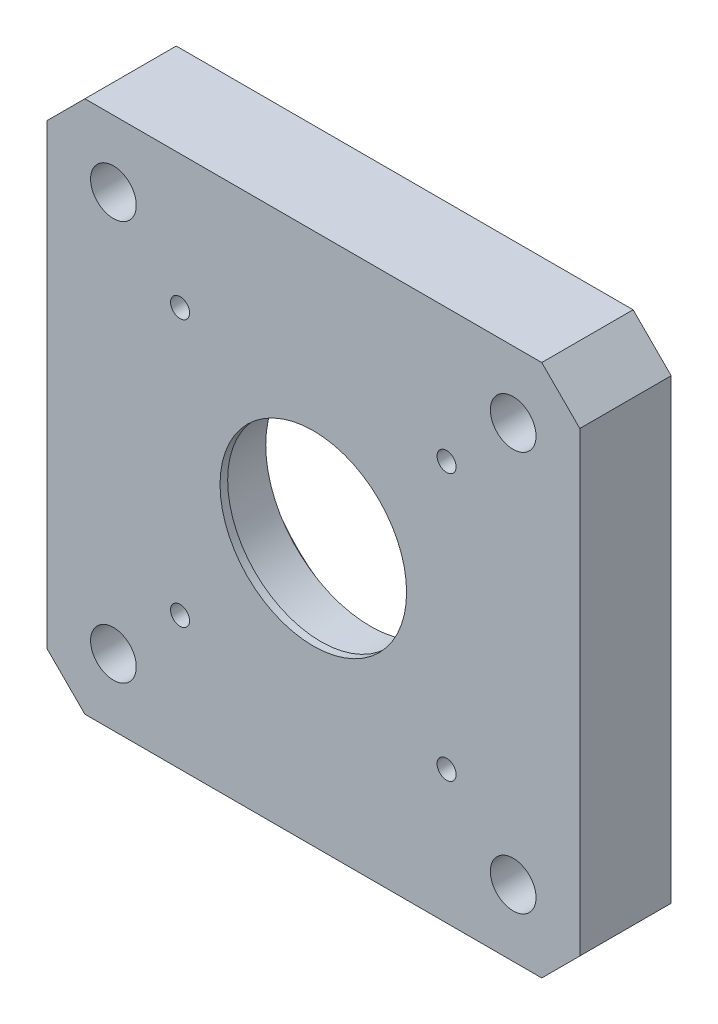
from build123d import *

# Parameters (mm, degrees)
SKETCH_1_W                    = 140
SKETCH_1_H                    = 140
EXTRUDE_1_DEPTH               = 24
SKETCH_2_R                    = 27.5
CUT_EXTRUDE_1_DEPTH           = 22
SKETCH_3_R                    = 24.5
CUT_EXTRUDE_2_DEPTH           = 102.410058673
HOLE_WIZARD_M10_1_D           = 12
HOLE_WIZARD_M10_1_CBORE_D     = 18
HOLE_WIZARD_M10_1_CBORE_DEPTH = 10.6
CHAMFER_1_SIZE                = 10
HOLE_WIZARD_M6_1_D            = 5
SKETCH_11_R                   = 40
CUT_EXTRUDE_3_DEPTH           = 9


with BuildPart() as part:
    # 草图1 → 凸台-拉伸1 (new body)
    with BuildSketch(Plane.XY):
        Rectangle(SKETCH_1_W, SKETCH_1_H)
    extrude(amount=EXTRUDE_1_DEPTH)

    # 草图2 → 切除-拉伸1 (cut)
    with BuildSketch(Plane(origin=(0, 0, 0), x_dir=(-1, 0, 0), z_dir=(0, 0, -1))):
        Circle(SKETCH_2_R)
    extrude(amount=-CUT_EXTRUDE_1_DEPTH, mode=Mode.SUBTRACT)

    # 草图3 → 切除-拉伸2 (cut, through all)
    with BuildSketch(Plane(origin=(0, 0, 22), x_dir=(-1, 0, 0), z_dir=(0, 0, -1))):
        Circle(SKETCH_3_R)
    extrude(amount=-CUT_EXTRUDE_2_DEPTH, mode=Mode.SUBTRACT)

    # M10 六角凹头螺钉的柱形沉头孔1 (through all)
    with Locations(Plane(origin=(0, 0, 0), x_dir=(-1, 0, 0), z_dir=(0, 0, -1))):
        with Locations((-52.5, 52.5), (52.5, 52.5), (52.5, -52.5), (-52.5, -52.5)):
            CounterBoreHole(HOLE_WIZARD_M10_1_D / 2, HOLE_WIZARD_M10_1_CBORE_D / 2, HOLE_WIZARD_M10_1_CBORE_DEPTH)

    # 倒角1
    chamfer_1_edges = [part.edges().sort_by_distance(p)[0] for p in [
        (70, -70, 12),
        (-70, -70, 12),
        (-70, 70, 12),
        (70, 70, 12),
    ]]
    chamfer(chamfer_1_edges, length=CHAMFER_1_SIZE)

    # M6 螺纹孔1 (through all)
    with Locations(Plane(origin=(0, 0, 0), x_dir=(-1, 0, 0), z_dir=(0, 0, -1))):
        with Locations((-35, 35), (35, 35), (35, -35), (-35, -35), (0, 0)):
            Hole(HOLE_WIZARD_M6_1_D / 2)

    # 草图11 → 切除-拉伸3 (cut)
    with BuildSketch(Plane(origin=(0, 0, 0), x_dir=(-1, 0, 0), z_dir=(0, 0, -1))):
        Circle(SKETCH_11_R)
    extrude(amount=-CUT_EXTRUDE_3_DEPTH, mode=Mode.SUBTRACT)


solid = part.part
